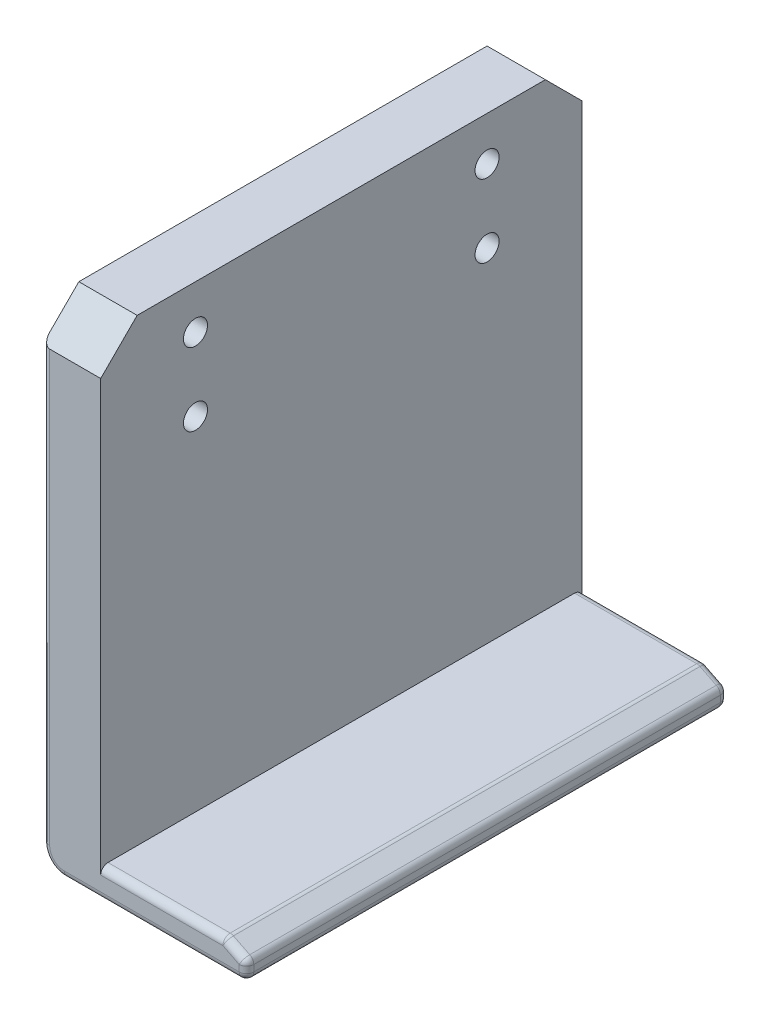
from build123d import *

# Parameters (mm, degrees)
EXTRUDE_1_DEPTH    = 33
CHAMFER_1_SIZE     = 1.5
CHAMFER_1_SIZE2    = 3
FILLET_1_R         = 1
CHAMFER_2_SIZE     = 5
FILLET_3_R         = 3
FILLET_4_R         = 1
HOLE_WIZARD_M4_2_D = 3.3


with BuildPart() as part:
    # 草图1 → 凸台-拉伸1 (new, symmetric)
    with BuildSketch(Plane.XY):
        Polygon((0, 67), (0, 0), (28, 0), (28, 4), (8, 4), (8, 67), align=None)
    extrude(amount=EXTRUDE_1_DEPTH, both=True)

    # 倒角1
    chamfer_1_edges = [part.edges().sort_by_distance(p)[0] for p in [
        (28, 4, 0),
    ]]
    chamfer_1_side = [part.faces().sort_by_distance(p)[0] for p in [
        (28, 2, 0),
    ]]
    chamfer(chamfer_1_edges, length=CHAMFER_1_SIZE, length2=CHAMFER_1_SIZE2, reference=chamfer_1_side[0])

    # 圆角1
    fillet_1_edges = [part.edges().sort_by_distance(p)[0] for p in [
        (28, 0, 0),
        (25, 4, 0),
        (28, 2.5, 0),
    ]]
    fillet(fillet_1_edges, radius=FILLET_1_R)

    # 倒角2
    chamfer_2_edges = [part.edges().sort_by_distance(p)[0] for p in [
        (4, 67, 33),
        (4, 67, -33),
    ]]
    chamfer(chamfer_2_edges, length=CHAMFER_2_SIZE)

    # 圆角3
    fillet_3_edges = [part.edges().sort_by_distance(p)[0] for p in [
        (0, 0, 0),
    ]]
    fillet(fillet_3_edges, radius=FILLET_3_R)

    # 圆角4
    fillet_4_edges = [part.edges().sort_by_distance(p)[0] for p in [
        (28, 1.440983006, -33),
        (28, 1.440983006, 33),
        (16.381966011, 4, -33),
        (26.329179607, 3.335410197, -33),
        (24.993684943, 3.973248989, -33),
        (27.850650808, 2.407697123, -33),
        (27.707106781, 0.292893219, -33),
        (26.329179607, 3.335410197, 33),
        (16.381966011, 4, 33),
        (24.993684943, 3.973248989, 33),
        (27.850650808, 2.407697123, 33),
        (27.707106781, 0.292893219, 33),
        (0, 32.5, 33),
        (0, 32.5, -33),
        (15, 0, -33),
        (15, 0, 33),
        (0.878679656, 0.878679656, -33),
        (0.878679656, 0.878679656, 33),
    ]]
    fillet(fillet_4_edges, radius=FILLET_4_R)

    # M4 螺纹孔2 (through all)
    with Locations(Plane.ZY):
        with Locations((-20, 61), (20, 61), (-20, 51), (20, 51)):
            Hole(HOLE_WIZARD_M4_2_D / 2)


solid = part.part
